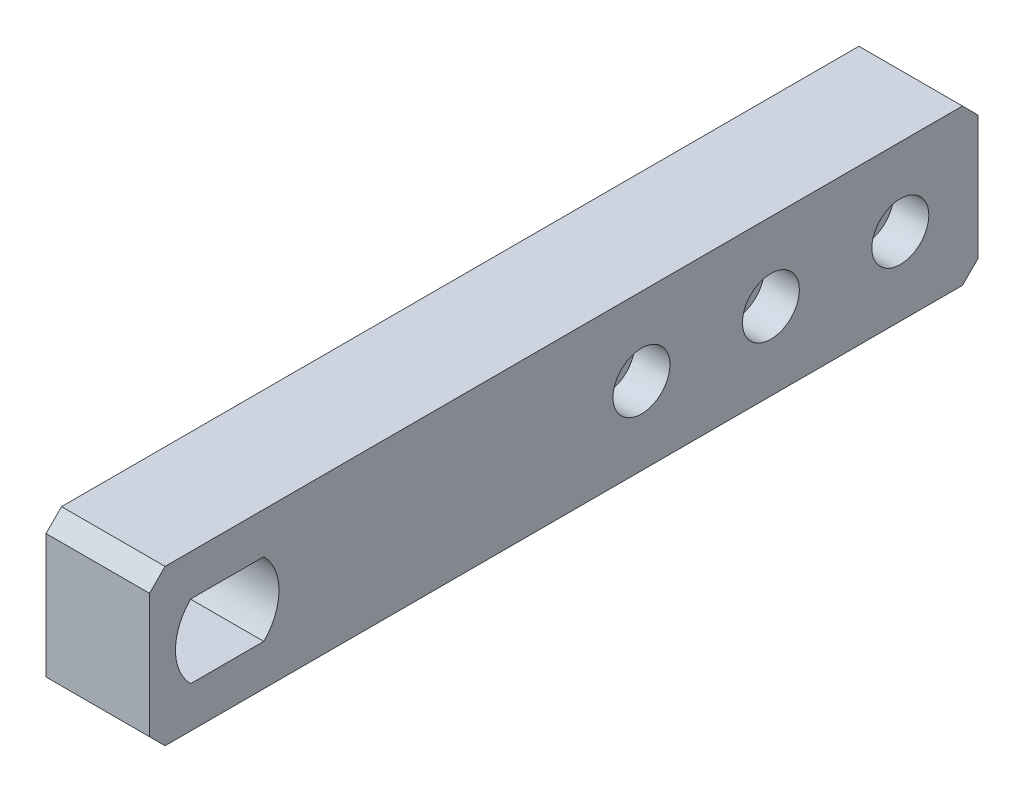
from build123d import *

# Parameters (mm, degrees)
SKETCH_1_W                = 160
SKETCH_1_H                = 30
EXTRUDE_1_DEPTH           = 20
CUT_EXTRUDE_1_DEPTH       = 84.815273071
HOLE_WIZARD_1_D           = 6.6
HOLE_WIZARD_1_DEPTH       = 38
HOLE_WIZARD_1_CBORE_D     = 11
HOLE_WIZARD_1_CBORE_DEPTH = 6.8
HOLE_WIZARD_1_TIP         = 1.982840043
CHAMFER_1_SIZE            = 3


with BuildPart() as part:
    # 草图1 → 凸台-拉伸1 (new body)
    with BuildSketch(Plane(origin=(0, 0, 0), x_dir=(0, 0, -1), z_dir=(1, 0, 0))):
        Rectangle(SKETCH_1_W, SKETCH_1_H)
    extrude(amount=EXTRUDE_1_DEPTH)

    # 草图2 → 切除-拉伸1 (cut, through all)
    with BuildSketch(Plane(origin=(20, 0, 0), x_dir=(0, 0, -1), z_dir=(1, 0, 0))):
        with BuildLine():
            Line((-72.062216973, 7.079907586), (-57.937783027, 7.079907586))
            ThreePointArc((-57.937783027, 7.079907586), (-55, 0), (-57.937783027, -7.079907586))
            Line((-57.937783027, -7.079907586), (-72.062216973, -7.079907586))
            ThreePointArc((-72.062216973, -7.079907586), (-75, 0), (-72.062216973, 7.079907586))
        make_face()
    extrude(amount=-CUT_EXTRUDE_1_DEPTH, mode=Mode.SUBTRACT)

    # 打孔尺寸(%根据)内六角圆柱头螺钉的类型1
    with Locations(Plane(origin=(20, 0, 0), x_dir=(0, 0, -1), z_dir=(1, 0, 0))):
        with Locations((15, 0), (40, 0), (65, 0)):
            CounterBoreHole(HOLE_WIZARD_1_D / 2, HOLE_WIZARD_1_CBORE_D / 2, HOLE_WIZARD_1_CBORE_DEPTH, depth=HOLE_WIZARD_1_DEPTH)
            with Locations((0, 0, -(HOLE_WIZARD_1_DEPTH + HOLE_WIZARD_1_TIP / 2))):  # 118° drill point
                Cone(0, HOLE_WIZARD_1_D / 2, HOLE_WIZARD_1_TIP, mode=Mode.SUBTRACT)

    # 倒角1
    chamfer_1_edges = [part.edges().sort_by_distance(p)[0] for p in [
        (10, -15, -80),
        (10, -15, 80),
        (10, 15, 80),
        (10, 15, -80),
    ]]
    chamfer(chamfer_1_edges, length=CHAMFER_1_SIZE)


solid = part.part
